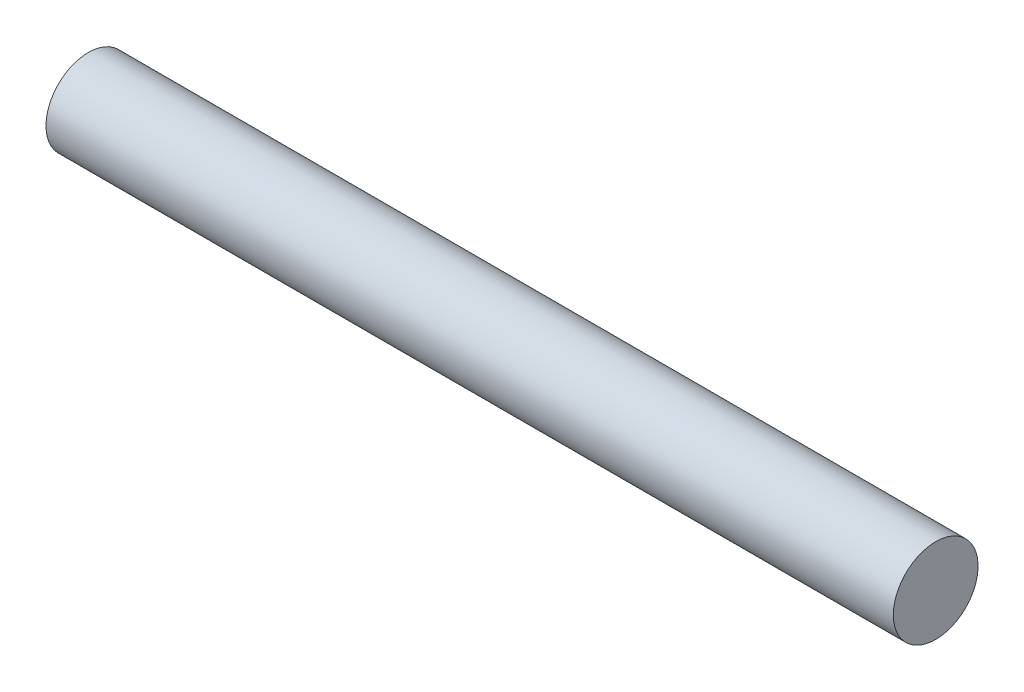
from build123d import *

# Parameters (mm, degrees)
SKETCH1_W = 30
SKETCH1_H = 1.5


with BuildPart() as part:
    # Sketch1 → Revolve1 (revolve)
    with BuildSketch(Plane.XY, mode=Mode.PRIVATE) as revolve1_sk:
        with Locations((15, 0.75)):
            Rectangle(SKETCH1_W, SKETCH1_H)
    revolve(revolve1_sk.sketch.rotate(Axis((0, 0, 0), (1, 0, 0)), 90), axis=Axis((0, 0, 0), (1, 0, 0)))


solid = part.part
